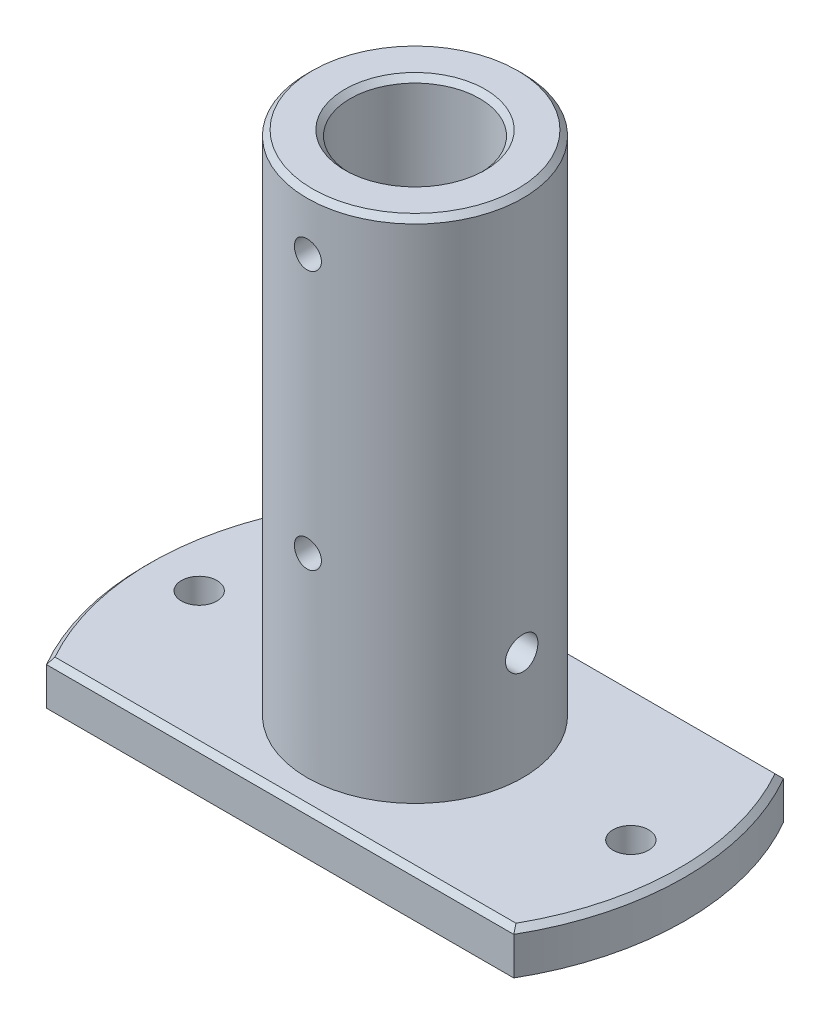
from build123d import *

# Parameters (mm, degrees)
CUT_EXTRUDE3_DEPTH    = 10
CHAMFER2_SIZE         = 0.5
M3_TAPPED_HOLE1_D     = 2.5
M3_TAPPED_HOLE1_DEPTH = 8.5
M3_TAPPED_HOLE1_TIP   = 0.751075774
M4_TAPPED_HOLE1_D     = 3.3
M4_TAPPED_HOLE1_DEPTH = 11.5
M4_TAPPED_HOLE1_TIP   = 0.991420021
SKETCH16_R            = 1.5
CUT_EXTRUDE4_DEPTH    = 26.5


with BuildPart() as part:
    # Sketch1 → Revolve1 (revolve)
    with BuildSketch(Plane.XY, mode=Mode.PRIVATE) as revolve1_sk:
        Polygon((10, 51), (10, 4), (25, 4), (25, 0), (6, 0), (6, 51), align=None)
    revolve(revolve1_sk.sketch.rotate(Axis((0, 57.582524272, 0), (0, -1, 0)), 90), axis=Axis((0, 57.582524272, 0), (0, -1, 0)))

    # Sketch9 → Cut-Extrude3 (cut)
    with BuildSketch(Plane(origin=(0, 4, 0), x_dir=(1, 0, 0), z_dir=(0, 1, 0))):
        with BuildLine():
            Line((-26.167728216, -12.5), (26.167728216, -12.5))
            ThreePointArc((26.167728216, -12.5), (0, -29), (-26.167728216, -12.5))
        make_face()
        with BuildLine():
            Line((-26.167728216, 12.5), (26.167728216, 12.5))
            ThreePointArc((26.167728216, 12.5), (0, 29), (-26.167728216, 12.5))
        make_face()
    extrude(amount=-CUT_EXTRUDE3_DEPTH, mode=Mode.SUBTRACT)

    # Chamfer2
    chamfer2_edges = [part.edges().sort_by_distance(p)[0] for p in [
        (-25, 4, 0),
        (0, 4, -12.5),
        (25, 4, 0),
        (0, 4, 12.5),
        (0, 51, -6),
        (0, 51, -10),
    ]]
    chamfer(chamfer2_edges, length=CHAMFER2_SIZE)

    # M3 Tapped Hole1
    with Locations(Plane(origin=(0, 22, 10), x_dir=(1, 0, 0), z_dir=(0, 0, 1))):
        with Locations((0, 0), (0, 24)):
            Hole(M3_TAPPED_HOLE1_D / 2, depth=M3_TAPPED_HOLE1_DEPTH)
            with Locations((0, 0, -(M3_TAPPED_HOLE1_DEPTH + M3_TAPPED_HOLE1_TIP / 2))):  # 118° drill point
                Cone(0, M3_TAPPED_HOLE1_D / 2, M3_TAPPED_HOLE1_TIP, mode=Mode.SUBTRACT)

    # M4 Tapped Hole1
    with Locations(Plane(origin=(-20, 0, 0), x_dir=(0, 0, -1), z_dir=(0, -1, 0))):
        with Locations((0, 0), (0, 40)):
            Hole(M4_TAPPED_HOLE1_D / 2, depth=M4_TAPPED_HOLE1_DEPTH)
            with Locations((0, 0, -(M4_TAPPED_HOLE1_DEPTH + M4_TAPPED_HOLE1_TIP / 2))):  # 118° drill point
                Cone(0, M4_TAPPED_HOLE1_D / 2, M4_TAPPED_HOLE1_TIP, mode=Mode.SUBTRACT)

    # Sketch16 → Cut-Extrude4 (cut, symmetric)
    with BuildSketch(Plane(origin=(0, 0, 0), x_dir=(0, 0, -1), z_dir=(1, 0, 0))):
        with Locations((0, 14)):
            Circle(SKETCH16_R)
    extrude(amount=CUT_EXTRUDE4_DEPTH, both=True, mode=Mode.SUBTRACT)


solid = part.part
